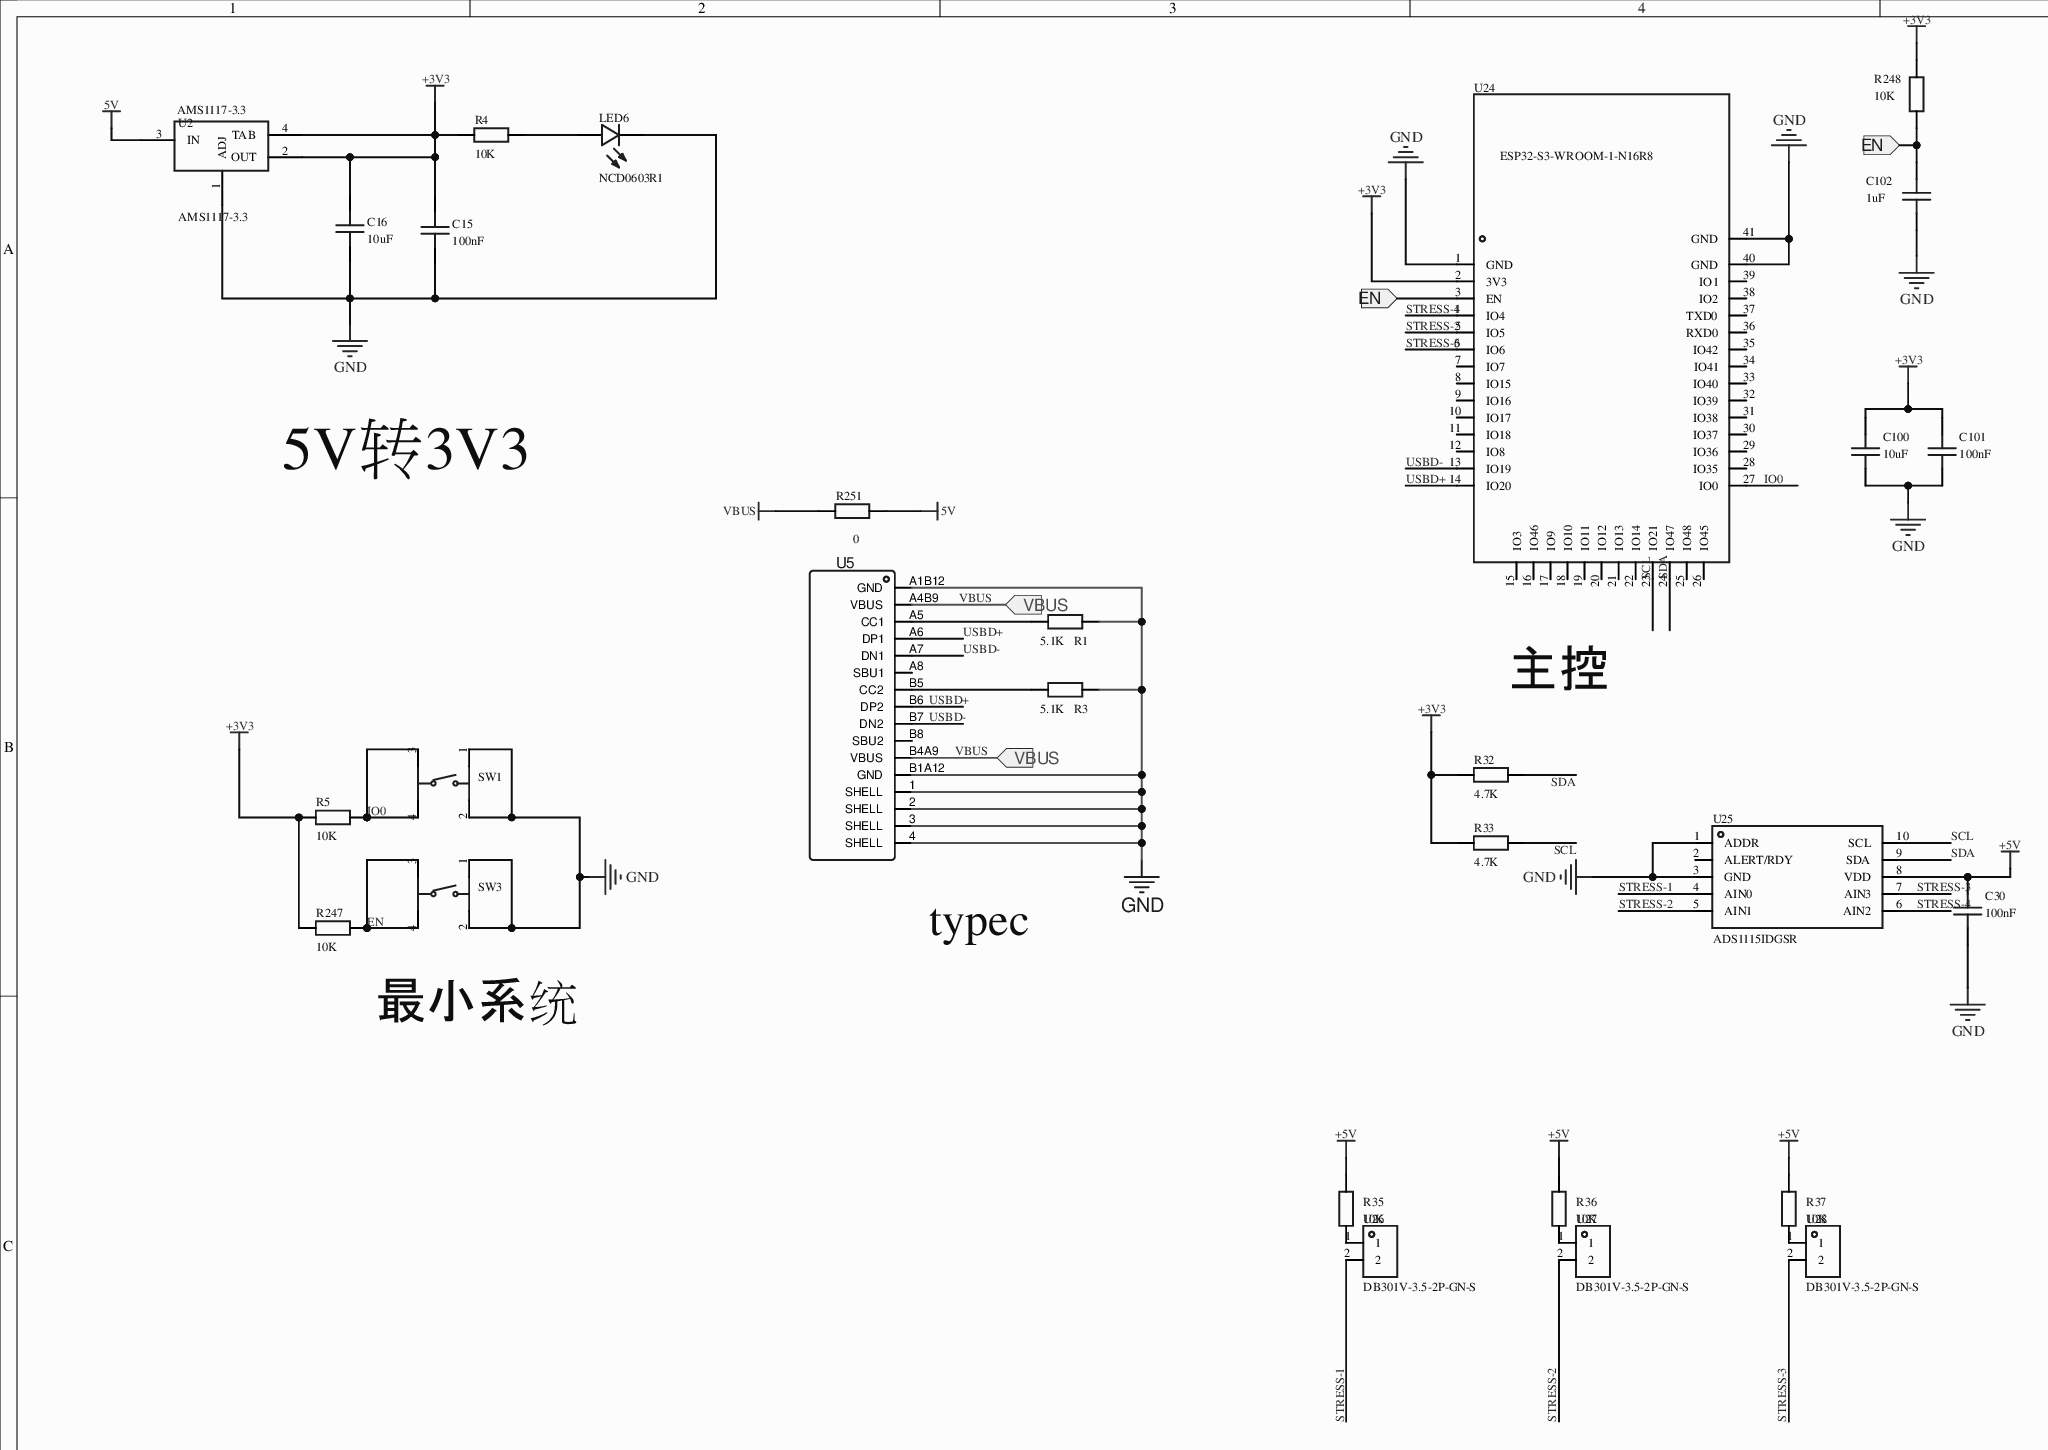
[diagram p0: MISC51586-2.schdoc]
# Altium project MISC51586-3.PrjPcb
1 sheet, 28 parts. Net scope: flat (ports and power ports of the same name join across sheets).
Board file: MISC51586.pcbdoc

## Sheet MISC51586-2.schdoc
size 420 x 297 mm; Version: V1.0; @Project Name: MISC51586; @Page Count: 1; @Update Date: 2025-03-15; @Create Date: 2025-03-15; @Schematic Name: MISC51586; @Page No: 1; @Board Name: MISC51586; @Create Time: 12:56:04; @Update Time: 12:56:10

### Parts
C15  100nF  [C0402]
C16  10uF  [C0402]
C30  100nF  [C0603]
C100  10uF  [C0402]
C101  100nF  [C0402]
C102  1uF  [C0402]
LED6  NCD0603R1  [LED0603-RD_RED]
R1  5.1K  [r0402]
R3  5.1K  [r0402]
R4  10K  [r0402]
R5  10K  [r0402]
R32  value 4.7K  [R0603]  (hidden comment: Res_0603)
R33  value 4.7K  [R0603]  (hidden comment: Res_0603)
R35  value 10K  [R0603]  (hidden comment: Res_0603)
R36  value 10K  [R0603]  (hidden comment: Res_0603)
R37  value 10K  [R0603]  (hidden comment: Res_0603)
R247  10K  [r0402]
R248  value 10K  [r0402]
R251  0  [r0402]
SW1  TS-1089S-02526  [SW-SMD_4P-L4.2-W3.3-P2.15-LS5.1]  (value not drawn)
SW3  TS-1089S-02526  [SW-SMD_4P-L4.2-W3.3-P2.15-LS5.1]  (value not drawn)
U2  AMS1117-3.3  [sot-223(gd32)]
U5  TYPE-C16P  [USB-C-SMD_TYPE-C16PIN-SHOUHAN]  (value not drawn)
U24  ESP32-S3-WROOM-1-N16R8  [WIRELM-SMD_ESP32-S3-WROOM-1]
U25  ADS1115IDGSR  [MSOP-10_L3.0-W3.0-P0.50-LS5.0-BL]
U26  DB301V-3.5-2P-GN-S  [CONN-TH_DB301V-3.5-2P-GN]
U27  DB301V-3.5-2P-GN-S  [CONN-TH_DB301V-3.5-2P-GN]
U28  DB301V-3.5-2P-GN-S  [CONN-TH_DB301V-3.5-2P-GN]

### Ports
EN (in), VBUS (in)

### Nets
5V: R251.2 U2.3(IN)
+3V3: C15.2 C16.2 C100.2 C101.2 R4.1 R5.1 R32.2 R33.2 R247.1 R248.2 U2.2(OUT) U2.4(TAB) U24.2(3V3)
+5V: C30.2 R35.2 R36.2 R37.2 U25.8(VDD)
GND: C15.1 C16.1 C30.1 C100.1 C101.1 C102.1 LED6.1(K) R1.2 R3.2 SW1.1 SW1.2 SW3.1 SW3.2 U2.1(ADJ) U5.1(SHELL) U5.2(SHELL) U5.3(SHELL) U5.4(SHELL) U5.A1B12(GND) U5.B1A12(GND) U24.1(GND) U24.40(GND) U24.41(GND) U25.1(ADDR) U25.3(GND)
VBUS: R251.1 U5.A4B9(VBUS) U5.B4A9(VBUS) ; port VBUS
EN: R247.2 SW3.3 SW3.4
IO0: R5.2 SW1.3 SW1.4 U24.27(IO0)
SCL: R33.1 U24.23(IO21) U25.10(SCL)
SDA: R32.1 U24.24(IO47) U25.9(SDA)
STRESS-1: U24.4(IO4) U25.4(AIN0) U26.2
STRESS-2: U24.5(IO5) U25.5(AIN1) U27.2
STRESS-3: U24.6(IO6) U25.7(AIN3) U28.2
STRESS-4: U25.6(AIN2)
USBD+: U5.A6(DP1) U5.B6(DP2) U24.14(IO20)
USBD-: U5.A7(DN1) U5.B7(DN2) U24.13(IO19)
NetC102_2: C102.2 R248.1 U24.3(EN) ; port EN
NetLED6_2: LED6.2(A) R4.2
NetR1_1: R1.1 U5.A5(CC1)
NetR3_1: R3.1 U5.B5(CC2)
NetR35_1: R35.1 U26.1
NetR36_1: R36.1 U27.1
NetR37_1: R37.1 U28.1

Not connected (* = marked no-connect by the designer): U5 A8(SBU1)* B8(SBU2)*; U24 7(IO7) 8(IO15) 9(IO16) 10(IO17) 11(IO18) 12(IO8) 15(IO3) 16(IO46) 17(IO9) 18(IO10) 19(IO11) 20(IO12) 21(IO13)* 22(IO14)* 25(IO48)* 26(IO45)* 28(IO35)* 29(IO36)* 30(IO37)* 31(IO38)* 32(IO39)* 33(IO40)* 34(IO41)* 35(IO42)* 36(RXD0)* 37(TXD0)* 38(IO2)* 39(IO1)*; U25 2(ALERT/RDY)*

### Notes on the sheet
- 5V转3V3
- 主控
- (near U5) typec
- 最小系统

### Library data of the parts
C15 C16 = CAP_0402: ConvertToPcb: yes; SymbolName: CapAcitance; ModelId: 36a51122f27c49738f86b3bfa98863e0; ModelName: C0402_L1.0-W0.5-H0.5; ModelTransform: 39.37,19.685,0,0,0,0,0,0,0; Device: CAP_0402; AddInBom: yes; Supplier Footprint: 0402; FootprintName: C0402
  C15: Value: 100nF
  C16: Value: 10uF
C30 C101 = 0603F104Z500CT_C83060: 容值:100nF;精度:-20%~+80%;额定电压:50V;材质(温度系数):Y5V;; Manufacturer: Walsin(华新科); Symbol: CapAcitance; Voltage Rated: 50V; Temperature Coefficient: Y5V; AddInBom: yes; ModelId: ac125912035d415993ca9572d50418b1; ModelName: C0603_L1.6-W0.8-H0.8; ModelTransform: 62.992,31.496,0,0,0,0,0,0,0; Value: 100nF; Device: 0603F104Z500CT_C83060; LCSC Part Name: 100nF -20%~+80% 50V; Supplier Part: C83060; Manufacturer Part: 0603F104Z500CT; JLCPCB Part Class: Extended Part; Datasheet: https://atta.szlcsc.com/upload/public/pdf/source/20161119/1479540179445.pdf; Supplier: LCSC; Tolerance: -20%~+80%; Supplier Footprint: 0603; ConvertToPcb: yes
  C30: FootprintName: C0603
  C101: FootprintName: C0402
C100 = CL10A105KB8NNNC: 容值:1uF;精度:±10%;额定电压:50V;材质(温度系数):X5R;; Manufacturer: SAMSUNG(三星); Symbol: CapAcitance; Tolerance: ±10%; Voltage Rated: 50V; Temperature Coefficient: X5R; AddInBom: yes; ModelId: ac125912035d415993ca9572d50418b1; ModelName: C0603_L1.6-W0.8-H0.8; ModelTransform: 62.992,31.496,0,0,0,0,0,0,0; Value: 10uF; Device: CL10A105KB8NNNC; LCSC Part Name: 1uF ±10% 50V; Supplier Part: C15849; Manufacturer Part: CL10A105KB8NNNC; JLCPCB Part Class: Basic Part; Datasheet: https://atta.szlcsc.com/upload/public/pdf/source/20160103/1457707679084.pdf; Supplier: LCSC; Supplier Footprint: 0603; ConvertToPcb: yes; FootprintName: C0402
C102 = CAP_0603: Symbol: C1210X7R475K630NT; ConvertToPcb: yes; ModelId: ac125912035d415993ca9572d50418b1; ModelName: C0603_L1.6-W0.8-H0.8; ModelTransform: 62.992,31.496,0,0,0,0,0,0,0; Value: 1uF; Device: CAP_0603; AddInBom: yes; Supplier Footprint: 0603; FootprintName: C0402
LED6 = NCD0603R1_C84263: 灯头类型:-;发光颜色:红色;正向电压(VF):1.6V~2.6V;功率:65mW;正向电流:20mA;主波长:615nm~630nm;二极管配置:独立二极管;透镜颜色:无色透明透镜;色温:-;发光强度:80mcd~220mcd;发光角度:130°;载带方式:-;工作温度:-30℃~+85℃;; Manufacturer: 国星光电; Symbol: FC-DA1608HRK-620D; AddInBom: yes; ModelId: 74041d3a270d435c8600a9ab9b7641c0; ModelTransform: 63.7794,31.496,0,0,0,0,0,0,0; Emitted Color: 红色; Power Dissipation: 65mW; Forward Current: 20mA; Diode Configuration: 独立二极管; Lens Color: 无色透明透镜; Viewing Angle: 130°; Device: NCD0603R1_C84263; Supplier: LCSC; Manufacturer Part: NCD0603R1; Supplier Part: C84263; LCSC Part Name: NCD0603R1; Supplier Footprint: 0603; Datasheet: https://atta.szlcsc.com/upload/public/pdf/source/20200820/C84263_DABC6A75E58F576973B407FDBA283D60.pdf; ConvertToPcb: yes; FootprintName: LED0603-RD_RED; ModelName: LED0603-RD_RED; Lamp Holder Type: -; Forward Voltage (VF): 1.6V~2.6V; Dominant Wavelength: 615nm~630nm; Peak Wavelength: -; Color Temperature: -; Luminous Intensity: 80mcd~220mcd; Mounting Sytle: -; Operating Temperature: -30℃~+85℃
R1 R3 R32 R33 R35-R37 = Res_0603: Symbol: 电阻; Check: true; ConvertToPcb: yes; ModelId: 8176a32bb9f4431db75ab5f6460c2416; ModelName: R0603_L1.6-W0.8-H0.5; ModelTransform: 63,31.5,20.1,0,0,0,0,0,0; Device: Res_0603; AddInBom: yes; Supplier Footprint: 0603
  R1 R3: Value: 5.1K; FootprintName: r0402
  R32 R33 R35-R37: FootprintName: R0603
R4 R5 R247 R251 = Res_0603: Symbol: 电阻; ConvertToPcb: yes; ModelId: fc143cca1e79419f9cd78b61e9279f08; ModelName: R0603; ModelTransform: 31.8897,63.7794,0,90,0,0,0,0,0; Device: Res_0603; AddInBom: yes; Supplier Footprint: 0603; FootprintName: r0402
  R4 R5 R247: Value: 10K
  R251: Value: 0
R248 = Res_0603: Symbol: 电阻; ConvertToPcb: yes; ModelId: 8176a32bb9f4431db75ab5f6460c2416; ModelName: R0603_L1.6-W0.8-H0.5; ModelTransform: 63,31.5,20.1,0,0,0,0,0,0; Device: Res_0603; AddInBom: yes; Supplier Footprint: 0603; FootprintName: r0402
SW1 SW3 = TS-1089S-02526: 电路结构:单刀单掷;按钮形状:椭圆形按钮;安装方式:立贴;开关长度:4.2mm;开关宽度:3.25mm;开关高度:2.5mm;触点电流:50mA;额定电压(DC):12V;带灯:-;机械寿命:-;; Manufacturer: XUNPU(讯普); AddInBom: yes; ModelId: 101da67941e24d4e9615179a94fc6132; ModelName: SW-SMD_4P-L4.2-W3.3-H2.5-P2.15-LS5.1; ModelTransform: 204.724,127.9525,0,0,0,0,0,0,0; Circuit: 单刀单掷; Actuator Style: 椭圆形按钮; Switch Length: 4.2mm; Switch Width: 3.25mm; Switch Height: 2.5mm; Contact Current: 50mA; Voltage Rating (DC): 12V; Symbol: TS-1089S-02526; Device: TS-1089S-02526; Supplier: LCSC; Supplier Part: C455282; Manufacturer Part: TS-1089S-02526; JLCPCB Part Class: 扩展库; LCSC Part Name: 4.2*3.25*2.5mm 立贴 轻触开关; Supplier Footprint: SMD,3.3x4.2mm; Datasheet: https://atta.szlcsc.com/upload/public/pdf/source/20191118/C455282_2E86A26A9CC4FEF4662951C4D45ED672.pdf; ConvertToPcb: yes; FootprintName: SW-SMD_4P-L4.2-W3.3-P2.15-LS5.1; Mounting Style: 立贴; With Lamp: -; Mechanical Life: -
U2 = AMS1117-3.3: AddInBom: yes; Device: AMS1117-3.3; ConvertToPcb: yes; SymbolName: AMS1117-3.3
U5 = TYPE-C16P: UART; Origin Footprint: USB-C-SMD_TYPE-C16PIN; Convert to PCB: yes; Check: true; ModelId: 30a76af2071c44dfb502f78fbd84e155; ModelTransform: 351.95,311.01,161.41,0,180,180,0,-45,-31; Device: TYPE-C16P; Symbol: TYPE-C16P; Add into BOM: yes; FootprintName: USB-C-SMD_TYPE-C16PIN-SHOUHAN; ModelName: USB-C-SMD_TYPE-C16PIN
U24 = ESP32-S3-WROOM-1-N16R8: Manufacturer: ESPRESSIF(乐鑫); Symbol: ESP32-S3-WROOM-1(N16R8); AddInBom: yes; ModelId: 481f5bdfc076422c9bb3c23c3ada9c17; ModelTransform: 708.73866,1003.97437,0,0,0,0,0,143.7,0; Device: ESP32-S3-WROOM-1-N16R8; Supplier: LCSC; Supplier Part: C2913202; Manufacturer Part: ESP32-S3-WROOM-1-N16R8; JLCPCB Part Class: 扩展库; LCSC Part Name: 通用型Wi-Fi+低功耗蓝牙MCU模组; Supplier Footprint: SMD,18x25.5mm; Datasheet: https://atta.szlcsc.com/upload/public/pdf/source/20220705/4E799F39581577F766659887F738A439.pdf; ConvertToPcb: yes; FootprintName: WIRELM-SMD_ESP32-S3-WROOM-1; ModelName: WIRELM-SMD_ESP32-S3-WROOM-1
U25 = ADS1115IDGSR: 接口:I2C;电源电压:2V~5.5V;采样率:860Hz;分辨率:16位;; Manufacturer: TI(德州仪器); AddInBom: yes; ModelId: b42a31f9e1fa4643bc7ea573b9bba7ed; ModelName: MSOP-10_L3.0-W3.0-H1.1-LS5.0-P0.50; ModelTransform: 118.11,196.85,0,0,0,0,0,0,0; Interface: I2C; differential input: 是; number of channels: 2; sampling frequency: 860Hz; resolution: 16位; Symbol: ADS1115IDGSR; Device: ADS1115IDGSR; LCSC Part Name: 具有内部基准、振荡器和可编程比较器且兼容 I2C 的ADS111x、超小型、低功耗 860SPS、16位ADC; SupplierPart: C37593; ManufacturerPart: ADS1115IDGSR; Supplier Footprint: VSSOP-10; Datasheet: https://www.ti.com/cn/lit/gpn/ads1115; Supplier: LCSC; ConvertToPcb: yes; FootprintName: MSOP-10_L3.0-W3.0-P0.50-LS5.0-BL; Supply Voltage: 2V~5.5V; Operating Temperature: -40℃~+125℃
U26-U28 = DB301V-3.5-2P-GN-S: 结构:1x2P;间距:3.5mm;颜色:绿色;安装方式:直插;额定电流:10A;额定电压:130V;排数:1;线规 - AWG:18~24;线规 - 平方毫米:0.5~1;每排PIN数:2;工作温度范围:-40℃~+105℃;; Manufacturer: DORABO(地博电气); AddInBom: yes; ModelId: 9d89c74026024576ad773a6ab9429b88; ModelTransform: 314.96,255.905,0,0,0,0,0,5.866,-137.795; Structure: 1x2P; Pitch: 3.5mm; Current Rating (Max): 10A; Voltage Rating (Max): 130V; Wire Gauge - AWG: 18~24; Wire Gauge - mm2: 0.5~1; Number of PINs Per Row: 2; Symbol: DB301V-3.5-2P-GN; Device: DB301V-3.5-2P-GN-S; LCSC Part Name: 3.5mm 1x2P 排数:1 每排P数:2 直插; SupplierPart: C695629; ManufacturerPart: DB301V-3.5-2P-GN-S; Supplier Footprint: 插件,P=3.5mm; JLCPCB Part Class: 扩展库; Datasheet: https://atta.szlcsc.com/upload/public/pdf/source/20230106/1B95616A85A883CA085E21635C8A8490.pdf; Supplier: LCSC; ConvertToPcb: yes; FootprintName: CONN-TH_DB301V-3.5-2P-GN; ModelName: CONN-TH_DB301V-3.5-2P-GN; Color: 绿色; Mounting Style: 直插; Number of Pins: 2P; Number of Rows: 1; Operating Temperature Range: -40℃~+105℃